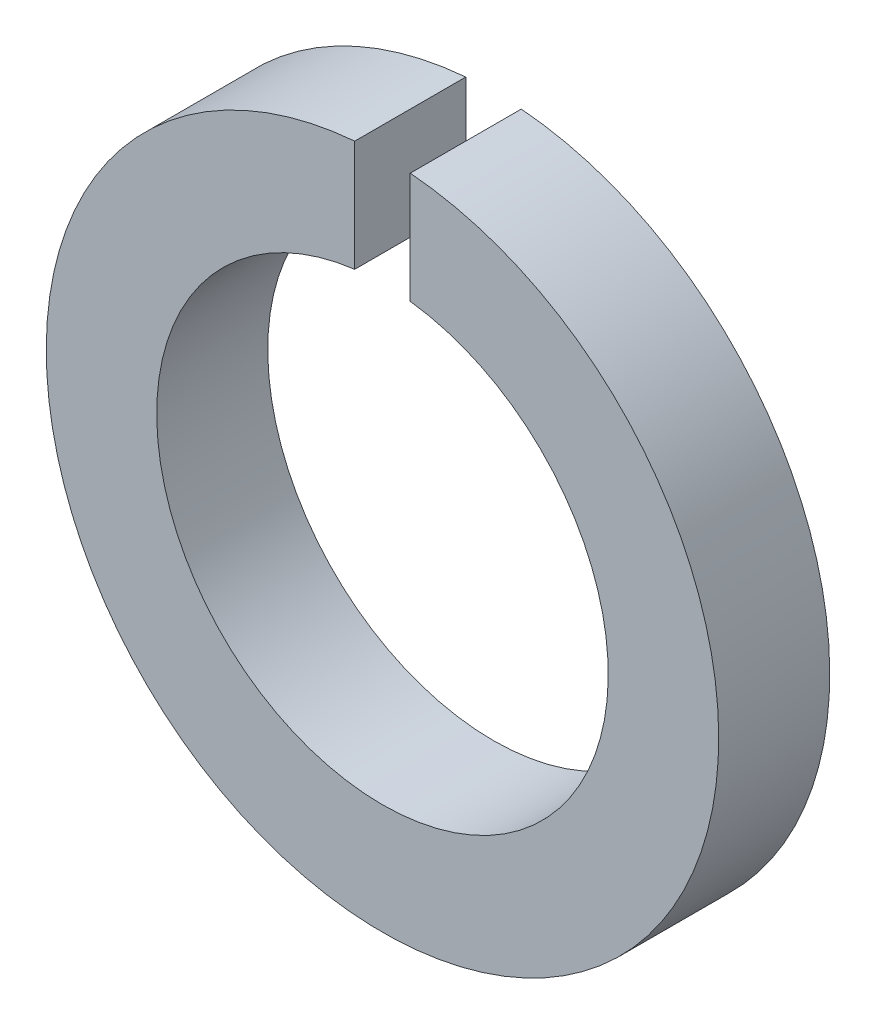
SolidWorks part; units mm, degrees
ref_plane "前视基准面" through (0, 0, 0) normal (0, 0, 1) x (1, 0, 0)
ref_plane "上视基准面" through (0, 0, 0) normal (0, 1, 0) x (1, 0, 0)
ref_plane "右视基准面" through (0, 0, 0) normal (1, 0, 0) x (0, 0, -1)
sketch "尺寸草图" plane through (0, 0, 0) normal (0, 0, 1) x (1, 0, 0)
  line L0 (0, 0) -> (0, 14.803) construction
  line L1 (-1.875, 22.6343) -> (-1.875, 15.1343)
  line L2 (1.875, 22.6343) -> (1.875, 15.1343)
  line L3 (0, 0) -> (7.5, 0) construction
  arc A0 (-1.875, 22.6343) -> (1.875, 22.6343) centre (0, 0) ccw
  arc A2 (-1.875, 15.1343) -> (1.875, 15.1343) centre (0, 0) ccw
  dimension "d" = 30.5
  dimension "m" = 3.75
  dimension "D4" = 1.875
  dimension "b" = 7.5
  dimension "s" = 7.5
extrude "拉伸1" add sketch "尺寸草图" along normal blind 7.5
